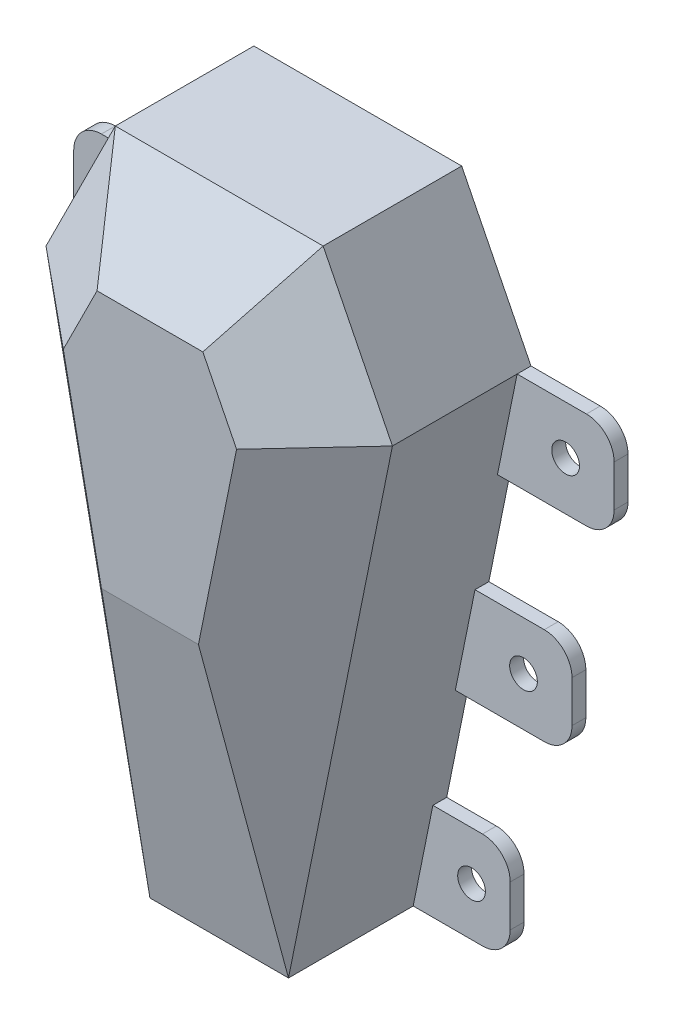
SolidWorks part; units mm, degrees
ref_plane "Front Plane" through (0, 0, 0) normal (0, 0, 1) x (1, 0, 0)
ref_plane "Top Plane" through (0, 0, 0) normal (0, 1, 0) x (1, 0, 0)
ref_plane "Right Plane" through (0, 0, 0) normal (1, 0, 0) x (0, 0, -1)
other "Configuration Table"
sketch "Sketch2" plane through (0, 0, 0) normal (0, 0, 1) x (1, 0, 0)
  line L0 (-50, 0) -> (50, 0)
  line L1 (50, 0) -> (125, 370)
  line L2 (125, 370) -> (75, 470)
  line L3 (75, 470) -> (-75, 470)
  line L4 (0, 470) -> (0, -66.4755) construction
  line L5 (-125, 370) -> (-75, 470)
  line L6 (-50, 0) -> (-125, 370)
  point P9 (0, 0)
  dimension "D1" = 470
  dimension "D2" = 250
  dimension "D3" = 150
  dimension "D4" = 100
  dimension "D5" = 100
extrude "Boss-Extrude1" add sketch "Sketch2" along normal blind 50 draft 50
sketch "Sketch5" plane through (0, 0, 0) normal (1, 0, 0) x (0, 0, -1)
  line L0 (-50, 225.9641) -> (0, 0)
  line L1 (-50, 59.5877) -> (-50, 361.7155) construction
  line L2 (0, 0) -> (-90.6553, 0)
  line L3 (-90.6553, 0) -> (-50, 225.9641)
extrude "Cut-Extrude2" cut sketch "Sketch5" against normal mid plane 876
shell "Shell1" thickness 5
sketch "Sketch6" plane through (0, 0, 0) normal (0, 0, -1) x (-1, 0, 0)
  line L0 (-116.844, 368.9185) -> (-70.1925, 462.2214) construction
  line L1 (-116.844, 368.9185) -> (-70.1925, 462.2214)
  line L2 (70.1925, 462.2214) -> (116.844, 368.9185) construction
  line L3 (70.1925, 462.2214) -> (116.844, 368.9185)
  line L4 (-70.1925, 462.2214) -> (70.1925, 462.2214) construction
  line L5 (-70.1925, 462.2214) -> (70.1925, 462.2214)
  line L6 (50, 0) -> (125, 370)
  line L7 (125, 370) -> (75, 470)
  line L8 (75, 470) -> (-75, 470)
  line L9 (-75, 470) -> (-125, 370)
  line L10 (-125, 370) -> (-50, 0)
  line L11 (-50, 0) -> (50, 0)
  line L12 (50, 0) -> (125, 370)
  line L13 (125, 370) -> (75, 470)
  line L14 (75, 470) -> (-75, 470)
  line L15 (-75, 470) -> (-125, 370)
  line L16 (-125, 370) -> (-50, 0)
  line L17 (-50, 0) -> (50, 0)
  line L18 (-46.7543, 23.143) -> (-116.844, 368.9185) construction
  line L19 (-46.7543, 23.143) -> (-116.844, 368.9185)
  line L20 (46.7543, 23.143) -> (-46.7543, 23.143) construction
  line L21 (46.7543, 23.143) -> (-46.7543, 23.143)
  line L22 (116.844, 368.9185) -> (46.7543, 23.143) construction
  line L23 (116.844, 368.9185) -> (46.7543, 23.143)
  dimension "D1" = 0
extrude "Boss-Extrude2" add sketch "Sketch6" along normal blind 100
sketch "Sketch7" plane through (0, 0, -100) normal (0, 0, -1) x (-1, 0, 0)
  line L0 (-46.7543, 23.143) -> (-116.844, 368.9185) construction
  line L1 (-46.7543, 23.143) -> (-116.844, 368.9185)
  line L2 (-70.1925, 462.2214) -> (-116.844, 368.9185) construction
  line L3 (-70.1925, 462.2214) -> (-116.844, 368.9185)
  line L4 (70.1925, 462.2214) -> (-70.1925, 462.2214) construction
  line L5 (70.1925, 462.2214) -> (-70.1925, 462.2214)
  line L6 (-50, 0) -> (50, 0)
  line L7 (50, 0) -> (125, 370)
  line L8 (125, 370) -> (75, 470)
  line L9 (75, 470) -> (-75, 470)
  line L10 (-75, 470) -> (-125, 370)
  line L11 (-125, 370) -> (-50, 0)
  line L12 (-50, 0) -> (50, 0)
  line L13 (50, 0) -> (125, 370)
  line L14 (125, 370) -> (75, 470)
  line L15 (75, 470) -> (-75, 470)
  line L16 (-75, 470) -> (-125, 370)
  line L17 (-125, 370) -> (-50, 0)
  line L18 (70.1925, 462.2214) -> (116.844, 368.9185) construction
  line L19 (70.1925, 462.2214) -> (116.844, 368.9185)
  line L20 (116.844, 368.9185) -> (46.7543, 23.143) construction
  line L21 (116.844, 368.9185) -> (46.7543, 23.143)
  line L22 (46.7543, 23.143) -> (-46.7543, 23.143) construction
  line L23 (46.7543, 23.143) -> (-46.7543, 23.143)
  dimension "D1" = 0
extrude "Boss-Extrude3" add sketch "Sketch7" against normal blind 5 contours L23 L1 L3 L5 L19 L21
ref_plane "Plane1" through (0, 0, -50) normal (0, 0, 1) x (1, 0, 0)
sketch "Sketch9" plane through (0, 0, -50) normal (0, 0, 1) x (1, 0, 0)
  line L0 (50, 0) -> (125, 370) construction
  line L1 (50, 0) -> (125, 370)
  line L2 (-125, 370) -> (-50, 0) construction
  line L3 (-125, 370) -> (-50, 0)
  line L4 (125, 370) -> (195, 370)
  line L5 (195, 370) -> (195, 300)
  line L6 (195, 300) -> (110.8108, 300)
  line L7 (94.5946, 220) -> (164.5946, 220)
  line L8 (164.5946, 220) -> (164.5946, 150)
  line L9 (164.5946, 150) -> (80.4054, 150)
  line L10 (50, 0) -> (120, 0)
  line L11 (120, 0) -> (120, 70)
  line L12 (120, 70) -> (64.1892, 70)
  circle A0 centre (160, 335) radius 10
  circle A1 centre (129.5946, 185) radius 10
  circle A2 centre (92.0946, 35) radius 10
  dimension "D8" = 20
  dimension "D9" = 20
  dimension "D10" = 20
  dimension "D1" = 70
  dimension "D2" = 70
  dimension "D3" = 70
  dimension "D4" = 70
  dimension "D5" = 70
  dimension "D6" = 70
  dimension "D7" = 80
extrude "Boss-Extrude4" add sketch "Sketch9" along normal blind 10 contours L6 L5 L4 L1 A0 | L9 L8 L7 L1 A1 | L11 L12 L1 L10 A2
cosmetic thread "Cosmetic Thread1" parameters "D2"=24
cosmetic thread "Cosmetic Thread2" parameters "D2"=24
cosmetic thread "Cosmetic Thread3" parameters "D2"=24
fillet "Fillet1" radius 20 2 edges at (195, 300, -45) (195, 370, -45)
fillet "Fillet2" radius 20 4 edges at (120, 70, -45) (120, 0, -45) (164.5946, 150, -45) (164.5946, 220, -45)
sketch "Sketch10" plane through (0, 0, -50) normal (0, 0, 1) x (1, 0, 0)
  line L0 (0, 488.8588) -> (0, -32.2905) construction
mirror "Mirror1" about plane through (0, 0, 0) normal (1, 0, 0) of "Boss-Extrude4"
fillet "Fillet3" radius 20 6 edges at (-120, 70, -45) (-120, 0, -45) (-164.5946, 150, -45) (-164.5946, 220, -45) (-195, 370, -45) (-195, 300, -45)
sketch "Sketch19" plane through (0, 0, -50) normal (0, 0, -1) x (-1, 0, 0)
  line L0 (94.5946, 220) -> (80.4054, 150)
  line L1 (80.4054, 150) -> (144.5946, 150)
  line L2 (144.5946, 150) -> (80.4054, 150) construction
  line L3 (94.5946, 220) -> (144.5946, 220)
  line L4 (164.5946, 200) -> (164.5946, 170)
  arc A0 (144.5946, 150) -> (164.5946, 170) centre (144.5946, 170) ccw construction
  arc A1 (164.5946, 200) -> (144.5946, 220) centre (144.5946, 200) ccw
  arc A2 (144.5946, 150) -> (164.5946, 170) centre (144.5946, 170) ccw
  circle A3 centre (129.5946, 185) radius 10
extrude "Boss-Extrude6" add sketch "Sketch19" along normal blind 50
sketch "Sketch35" plane through (0, 0, -50) normal (0, 0, -1) x (-1, 0, 0)
  line L0 (110.8108, 300) -> (175, 300)
  line L1 (94.5946, 220) -> (125, 370) construction
  line L2 (175, 300) -> (110.8108, 300) construction
  line L3 (125, 370) -> (175, 370)
  line L4 (195, 350) -> (195, 320)
  line L5 (195, 350) -> (195, 320) construction
  line L6 (125, 370) -> (110.8108, 300)
  arc A0 (175, 300) -> (195, 320) centre (175, 320) ccw construction
  circle A1 centre (160, 335) radius 10
  arc A2 (175, 370) -> (195, 350) centre (175, 350) cw
  arc A3 (175, 300) -> (195, 320) centre (175, 320) ccw
extrude "Boss-Extrude7" add sketch "Sketch35" along normal blind 50
sketch "Sketch36" plane through (0, 0, -50) normal (0, 0, -1) x (-1, 0, 0)
  line L0 (64.1892, 70) -> (50, 0)
  line L1 (50, 0) -> (100, 0)
  line L2 (64.1892, 70) -> (100, 70)
  line L3 (100, 70) -> (64.1892, 70) construction
  line L4 (120, 50) -> (120, 20)
  arc A0 (120, 50) -> (100, 70) centre (100, 50) ccw construction
  arc A1 (100, 70) -> (120, 50) centre (100, 50) cw
  arc A2 (120, 20) -> (100, 0) centre (100, 20) cw
  circle A3 centre (92.0946, 35) radius 10
extrude "Boss-Extrude8" add sketch "Sketch36" along normal blind 50
sketch "Sketch37" plane through (0, 0, -50) normal (0, 0, -1) x (-1, 0, 0)
  line L0 (-100, 70) -> (-64.1892, 70)
  line L1 (-64.1892, 70) -> (-50, 0)
  line L2 (-50, 0) -> (-100, 0)
  line L3 (-120, 20) -> (-120, 50) construction
  line L4 (-120, 50) -> (-120, 20)
  circle A0 centre (-92.0946, 35) radius 10
  arc A1 (-100, 0) -> (-120, 20) centre (-100, 20) cw
  arc A2 (-120, 20) -> (-100, 0) centre (-100, 20) ccw construction
  arc A3 (-100, 70) -> (-120, 50) centre (-100, 50) ccw
extrude "Boss-Extrude9" add sketch "Sketch37" along normal blind 50
sketch "Sketch38" plane through (0, 0, -50) normal (0, 0, -1) x (-1, 0, 0)
  line L0 (-144.5946, 220) -> (-94.5946, 220)
  line L1 (-125, 370) -> (-64.1892, 70) construction
  line L2 (-94.5946, 220) -> (-80.4054, 150)
  line L3 (-80.4054, 150) -> (-144.5946, 150)
  line L4 (-164.5946, 170) -> (-164.5946, 200)
  circle A0 centre (-129.5946, 185) radius 10
  arc A1 (-164.5946, 200) -> (-144.5946, 220) centre (-144.5946, 200) cw
  arc A2 (-164.5946, 170) -> (-144.5946, 150) centre (-144.5946, 170) ccw
extrude "Boss-Extrude10" add sketch "Sketch38" along normal blind 50
sketch "Sketch39" plane through (0, 0, -50) normal (0, 0, -1) x (-1, 0, 0)
  line L0 (-175, 370) -> (-125, 370)
  line L1 (-125, 370) -> (-110.8108, 300)
  line L2 (-110.8108, 300) -> (-175, 300)
  line L3 (-195, 320) -> (-195, 350)
  line L4 (-195, 350) -> (-195, 320) construction
  arc A0 (-175, 370) -> (-195, 350) centre (-175, 350) ccw construction
  arc A1 (-195, 320) -> (-175, 300) centre (-175, 320) ccw construction
  circle A2 centre (-160, 335) radius 10
  arc A3 (-175, 300) -> (-195, 320) centre (-175, 320) cw
  arc A4 (-195, 350) -> (-175, 370) centre (-175, 350) cw
extrude "Boss-Extrude11" add sketch "Sketch39" along normal blind 50
ref_plane "Plane6" through (0, 0, -40) normal (0, 0, 1) x (1, 0, 0)
sketch "Sketch45" plane through (0, 0, -40) normal (0, 0, 1) x (1, 0, 0)
  line L0 (-175, 370) -> (-125, 370)
  line L1 (-125, 370) -> (-110.8108, 300)
  line L2 (-125, 370) -> (-50, 0) construction
  line L3 (-175, 300) -> (-110.8108, 300) construction
  line L4 (-110.8108, 300) -> (-175, 300)
  line L5 (-195, 320) -> (-195, 350)
  arc A0 (-195, 320) -> (-175, 300) centre (-175, 320) ccw construction
  circle A1 centre (-160, 335) radius 10
  arc A2 (-195, 350) -> (-175, 370) centre (-175, 350) cw
  arc A3 (-195, 320) -> (-175, 300) centre (-175, 320) ccw
extrude "Cut-Extrude3" cut sketch "Sketch45" against normal blind 50
sketch "Sketch46" plane through (0, 0, -40) normal (0, 0, 1) x (1, 0, 0)
  line L0 (-144.5946, 220) -> (-94.5946, 220)
  line L1 (-94.5946, 220) -> (-80.4054, 150)
  line L2 (-80.4054, 150) -> (-144.5946, 150)
  line L3 (-164.5946, 170) -> (-164.5946, 200)
  line L4 (-164.5946, 200) -> (-164.5946, 170) construction
  arc A0 (-144.5946, 220) -> (-164.5946, 200) centre (-144.5946, 200) ccw construction
  arc A1 (-164.5946, 200) -> (-144.5946, 220) centre (-144.5946, 200) cw
  arc A2 (-164.5946, 170) -> (-144.5946, 150) centre (-144.5946, 170) ccw
extrude "Cut-Extrude4" cut sketch "Sketch46" against normal blind 50
sketch "Sketch47" plane through (0, 0, -40) normal (0, 0, 1) x (1, 0, 0)
  line L0 (-100, 70) -> (-64.1892, 70)
  line L1 (-125, 370) -> (-50, 0) construction
  line L2 (-50, 0) -> (-64.1892, 70) construction
  line L3 (-64.1892, 70) -> (-50, 0)
  line L4 (-50, 0) -> (-100, 0)
  line L5 (-120, 20) -> (-120, 50)
  arc A0 (-100, 70) -> (-120, 50) centre (-100, 50) ccw construction
  arc A1 (-120, 50) -> (-100, 70) centre (-100, 50) cw
  arc A2 (-100, 0) -> (-120, 20) centre (-100, 20) cw
extrude "Cut-Extrude5" cut sketch "Sketch47" against normal blind 50
sketch "Sketch49" plane through (0, 0, -40) normal (0, 0, 1) x (1, 0, 0)
  line L0 (125, 370) -> (175, 370)
  line L1 (125, 370) -> (175, 370) construction
  line L2 (125, 370) -> (110.8108, 300)
  line L3 (110.8108, 300) -> (175, 300)
  line L4 (195, 350) -> (195, 320)
  arc A0 (195, 350) -> (175, 370) centre (175, 350) ccw construction
  arc A1 (175, 370) -> (195, 350) centre (175, 350) cw
  arc A2 (195, 320) -> (175, 300) centre (175, 320) cw
extrude "Cut-Extrude6" cut sketch "Sketch49" against normal blind 50
sketch "Sketch50" plane through (0, 0, -40) normal (0, 0, 1) x (1, 0, 0)
  line L0 (94.5946, 220) -> (144.5946, 220)
  line L1 (164.5946, 200) -> (164.5946, 170)
  line L2 (94.5946, 220) -> (80.4054, 150)
  line L3 (80.4054, 150) -> (144.5946, 150)
  line L4 (144.5946, 150) -> (80.4054, 150) construction
  arc A0 (164.5946, 200) -> (144.5946, 220) centre (144.5946, 200) ccw construction
  arc A1 (144.5946, 150) -> (164.5946, 170) centre (144.5946, 170) ccw construction
  arc A2 (144.5946, 220) -> (164.5946, 200) centre (144.5946, 200) cw
  arc A3 (164.5946, 170) -> (144.5946, 150) centre (144.5946, 170) cw
extrude "Cut-Extrude7" cut sketch "Sketch50" against normal blind 50
sketch "Sketch51" plane through (0, 0, -40) normal (0, 0, 1) x (1, 0, 0)
  line L0 (100, 70) -> (64.1892, 70)
  line L1 (64.1892, 70) -> (50, 0)
  line L2 (50, 0) -> (100, 0)
  line L3 (120, 50) -> (120, 20)
  arc A0 (100, 70) -> (120, 50) centre (100, 50) cw
  arc A1 (120, 20) -> (100, 0) centre (100, 20) cw
extrude "Cut-Extrude8" cut sketch "Sketch51" against normal blind 50
